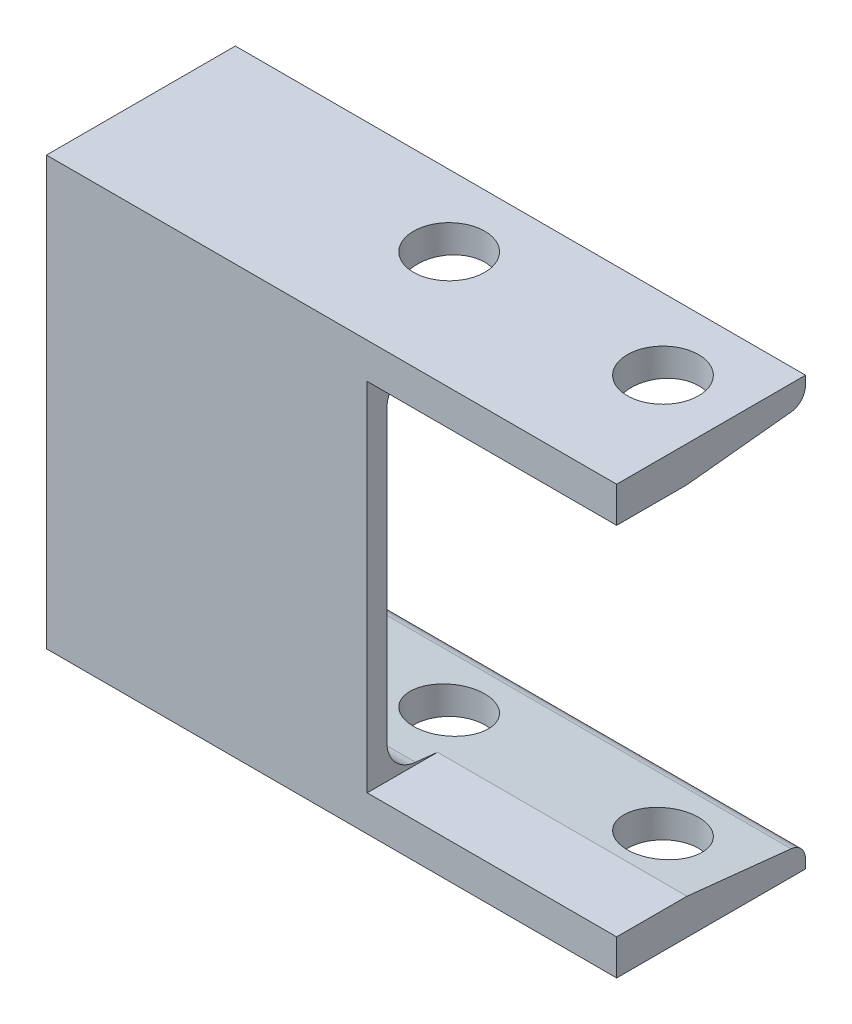
SolidWorks part; units mm, degrees
material "普通碳钢"
ref_plane "前视基准面" through (0, 0, 0) normal (0, 0, 1) x (1, 0, 0)
ref_plane "上视基准面" through (0, 0, 0) normal (0, 1, 0) x (1, 0, 0)
ref_plane "右视基准面" through (0, 0, 0) normal (1, 0, 0) x (0, 0, -1)
sketch3d "3D草图1"
  line L0 (0, 0, 0) -> (160, 0, 0)
  dimension "D1" = 160
other "C 槽 12(1)"
ref_plane "基准面1" through (0, 0, 0) normal (1, 0, 0) x (0, 0, -1)
sketch "Sketch11" plane through (0, 0, 0) normal (1, 0, 0) x (0, 0, -1)
  line L0 (53, 120) -> (0, 120)
  line L1 (53, 0) -> (0, 0)
  line L2 (0, 120) -> (0, 0)
  line L3 (-9.5694, 60) -> (49.7414, 60) construction
  line L4 (5.5, 100.4001) -> (5.5, 19.5999)
  line L5 (53, 0) -> (53, 2.452)
  line L6 (53, 120) -> (53, 117.548)
  line L7 (13.5592, 10.6492) -> (48.9704, 6.9273)
  line L17 (13.5592, 109.3508) -> (48.9704, 113.0727)
  arc A0 (48.9704, 113.0727) -> (53, 117.548) centre (48.5, 117.548) ccw
  arc A1 (48.9704, 6.9273) -> (53, 2.452) centre (48.5, 2.452) cw
  arc A2 (5.5, 19.5999) -> (13.5592, 10.6492) centre (14.5, 19.5999) ccw
  arc A10 (5.5, 100.4001) -> (13.5592, 109.3508) centre (14.5, 100.4001) cw
  point P6 (0, 0)
  point P8 (0, 60)
  point P9 (5.5, 25.8841)
  point P10 (26.5, 120)
  point P13 (53, 113.4962)
  point P14 (29.25, 111)
  point P19 (5.5, 60)
sketch "草图2" plane through (0, 0, 0) normal (0, 0, 1) x (1, 0, 0)
  line L0 (190, 60) -> (160, 60) construction
  line L1 (90, 110) -> (190, 110)
  line L2 (90, 110) -> (90, 10)
  line L3 (90, 10) -> (190, 10)
  line L4 (190, 110) -> (190, 10)
  line L5 (160, 120) -> (160, 0) construction
  line L6 (0, 120) -> (0, 0) construction
  dimension "D1" = 100
  dimension "D2" = 90
  dimension "D3" = 100
extrude "切除-拉伸1" cut sketch "草图2" against normal blind 40
sketch "草图3" plane through (0, 0, 0) normal (0, -1, 0) x (1, 0, 0)
  line L0 (0, -33) -> (160, -33) construction
  line L1 (0, 0) -> (0, -53) construction
  line L2 (160, 0) -> (160, -53) construction
  line L3 (0, 0) -> (160, 0) construction
  circle A0 centre (140, -33) radius 10
  circle A1 centre (80, -33) radius 10
  dimension "D1" = 20
  dimension "D2" = 20
  dimension "D3" = 33
  dimension "D4" = 80
  dimension "D5" = 60
extrude "切除-拉伸2" cut sketch "草图3" against normal up to surface (120 mm away) up to face at (80, 120, -26.5)
equation "\"RI@Sketch11\" = \"D1@Sketch11\""
equation "\"D3@Sketch11\" =  ( \"BF@Sketch11\" - \"D6@Sketch11\" )  / 2"
